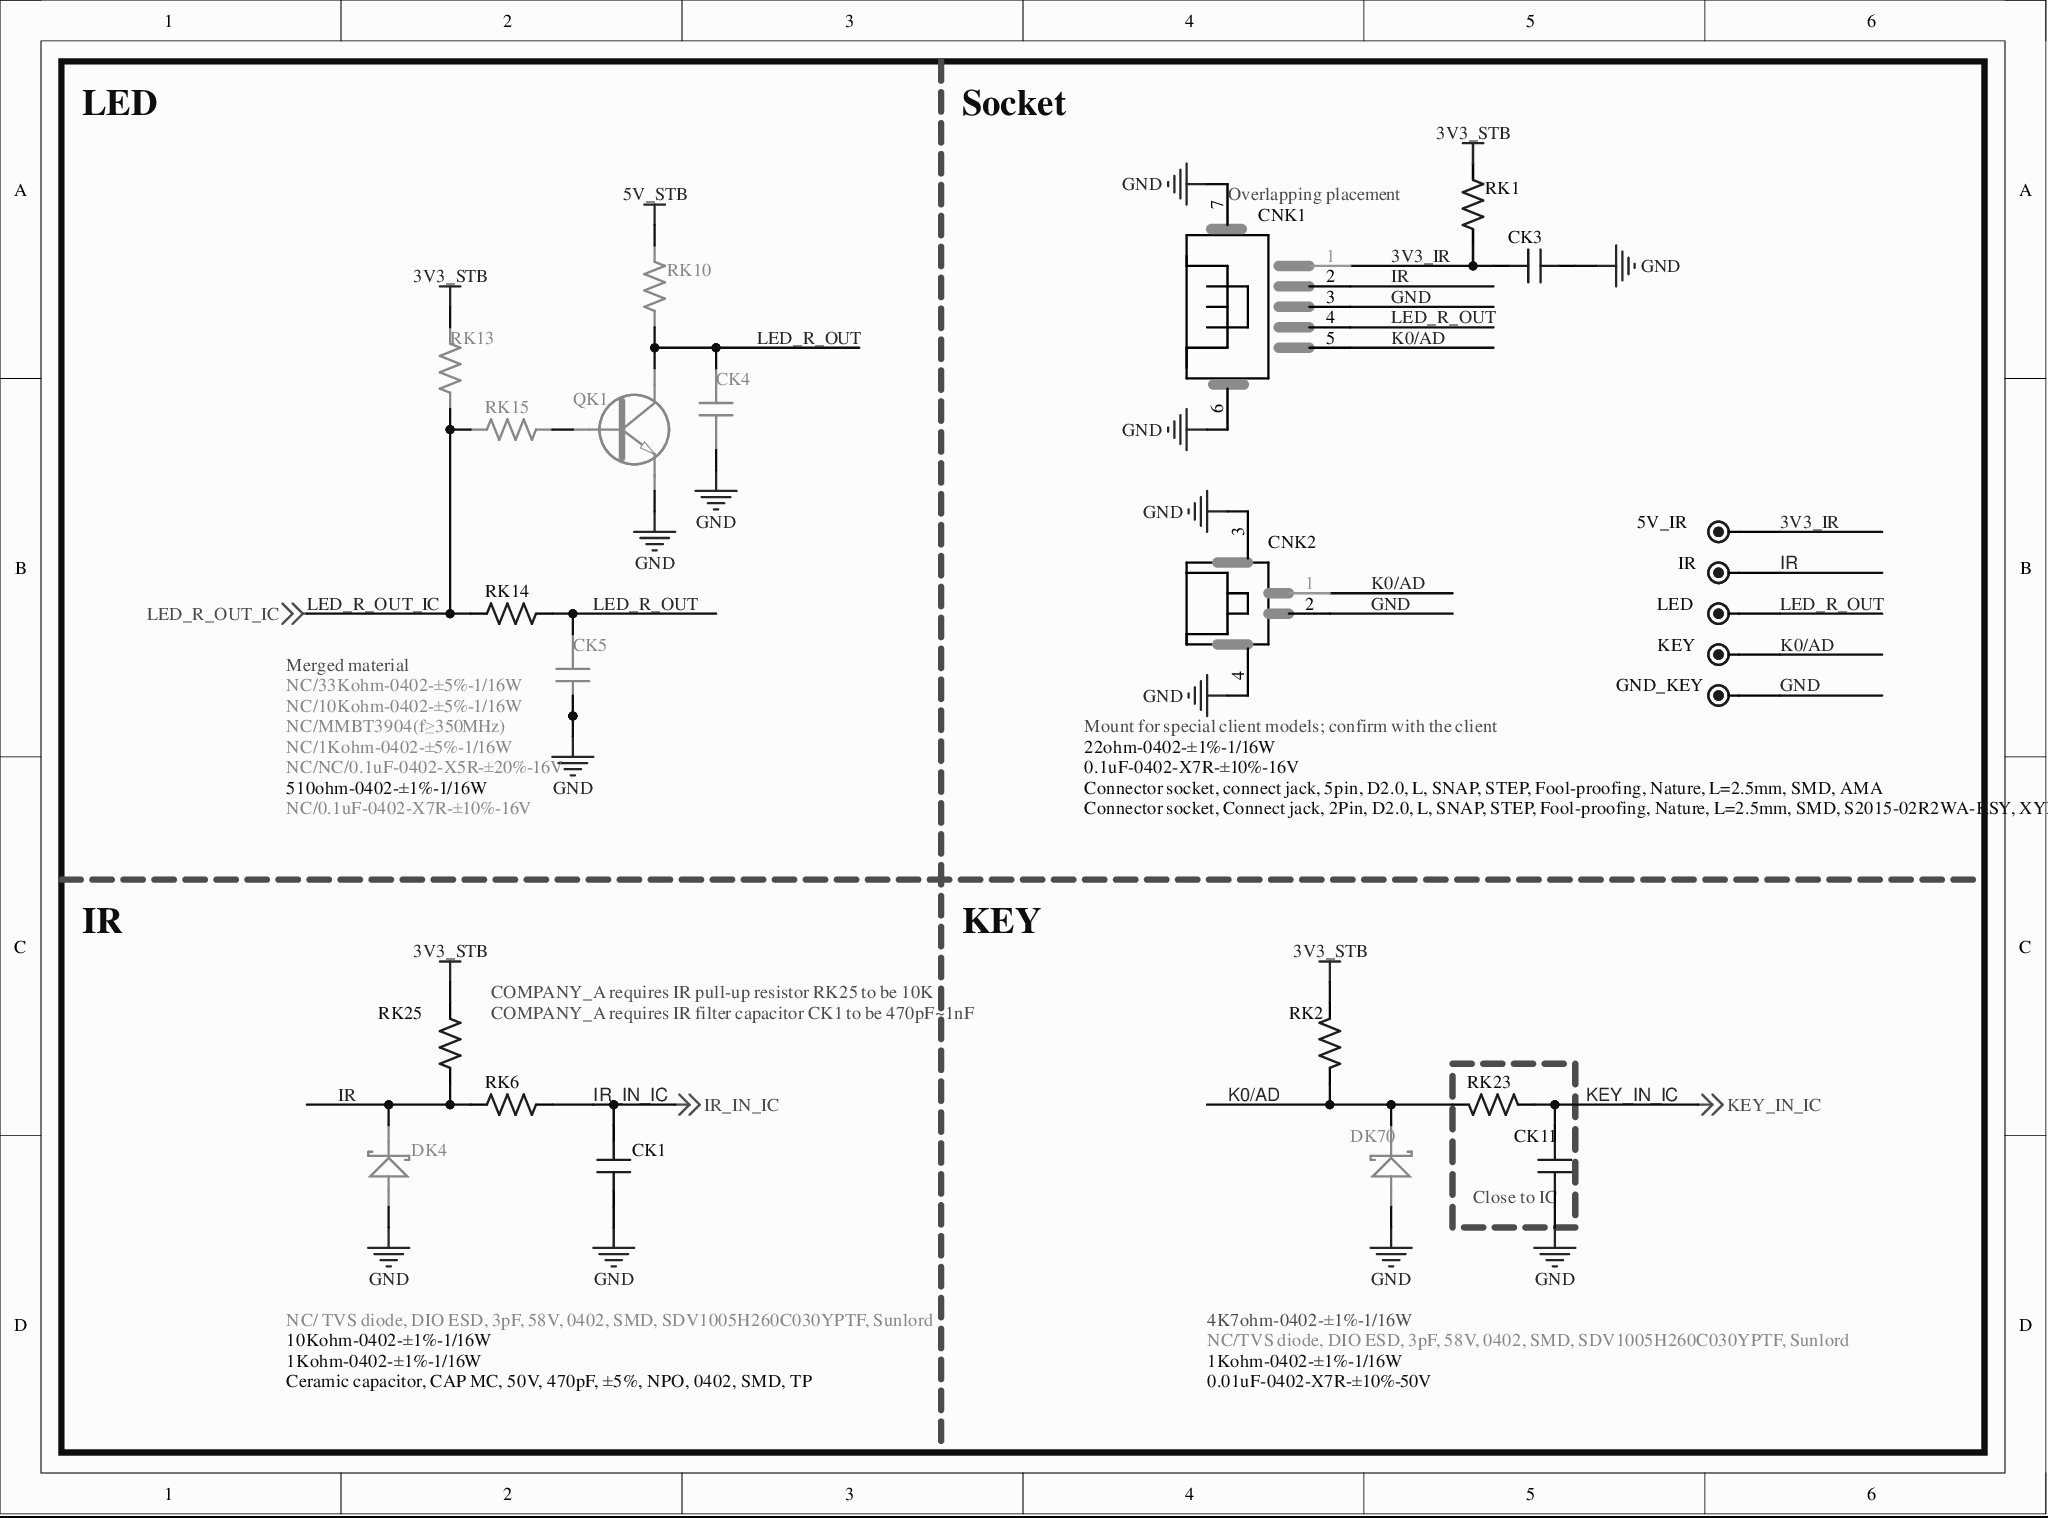
[diagram p0: MISC105950-37.SchDoc]
# Altium project MISC105950-48.PrjPCB (part 5 of 8)

## Sheet MISC105950-37.SchDoc
size 254 x 187 mm

### Parts
5V_IR  DM0  [TP]  (value not drawn)
CK1  Ceramic capacitor, CAP MC, 50V, 470pF, ±5%, NPO, 0402, SMD, TP  [C0402]
CK3  0.1uF-0402-X7R-±10%-16V  [C0402]
CK4  NC/NC/0.1uF-0402-X5R-±20%-16V  [C0402]
CK5  NC/0.1uF-0402-X7R-±10%-16V  [C0402]
CK11  0.01uF-0402-X7R-±10%-50V  [C0402]
CNK1  Connector socket, connect jack, 5pin, D2.0, L, SNAP, STEP, Fool-proofing, Nature, L=2.5mm, SMD, AMA  [SIP5H/2.0S-4]
CNK2  Connector socket, Connect jack, 2Pin, D2.0, L, SNAP, STEP, Fool-proofing, Nature, L=2.5mm, SMD, S2015-02R2WA-KSY, XYDT  [SIP2H/2.0S-3]
DK4  NC/ TVS diode, DIO ESD, 3pF, 58V, 0402, SMD, SDV1005H260C030YPTF, Sunlord  [DIODE-S0402]
DK70  NC/TVS diode, DIO ESD, 3pF, 58V, 0402, SMD, SDV1005H260C030YPTF, Sunlord  [DIODE-S0402]
GND_KEY  DM0  [TP]  (value not drawn)
IR  DM0  [TP]  (value not drawn)
KEY  DM0  [TP]  (value not drawn)
LED  DM0  [TP]  (value not drawn)
QK1  NC/MMBT3904(f≥350MHz)  [SOT-23]
RK1  22ohm-0402-±1%-1/16W  [R0402]
RK2  4K7ohm-0402-±1%-1/16W  [R0402]
RK6  1Kohm-0402-±1%-1/16W  [R0402]
RK10  NC/1Kohm-0402-±5%-1/16W  [R0402]
RK13  NC/33Kohm-0402-±5%-1/16W  [R0402]
RK14  510ohm-0402-±1%-1/16W  [R0402]
RK15  NC/10Kohm-0402-±5%-1/16W  [R0402]
RK23  1Kohm-0402-±1%-1/16W  [R0402]
RK25  10Kohm-0402-±1%-1/16W  [R0402]

### Blocks framed on the sheet
Close to IC: CK11 RK23

### Nets
3V3_STB: RK1.1 RK2.2 RK13.2 RK25.2
5V_STB: RK10.2
GND: CK1.1 CK3.2 CK4.1 CK5.1 CK11.2 CNK1.3 CNK1.6 CNK1.7 CNK2.2 CNK2.3 CNK2.4 DK4.A DK70.A GND_KEY.1 QK1.E
3V3_IR: 5V_IR.1 CK3.1 CNK1.1 RK1.2
IR: CNK1.2 DK4.K IR.1 RK6.1 RK25.1
IR_IN_IC: CK1.2 RK6.2 ; off-sheet IR_IN_IC
K0/AD: CNK1.5 CNK2.1 DK70.K KEY.1 RK2.1 RK23.2
KEY_IN_IC: CK11.1 RK23.1 ; off-sheet KEY_IN_IC
LED_R_OUT: CK4.2 CK5.2 CNK1.4 LED.1 QK1.C RK10.1 RK14.2
LED_R_OUT_IC: RK13.1 RK14.1 RK15.1 ; off-sheet LED_R_OUT_IC
NetQK1_B: QK1.B RK15.2

### Notes on the sheet
- LED
- Socket
- (near CNK1) Overlapping placement
- (near RK14) Merged material
- (near CNK2) Mount for special client models; confirm with the client
- IR
- KEY
- (near RK25) COMPANY_A requires IR filter capacitor CK1 to be 470pF
  nF
- (near RK25) COMPANY_A requires IR pull-up resistor RK25 to be 10K

### Library data of the parts
5V_IR GND_KEY IR KEY LED = TEST
CK1 = 22pF-0402-NPO-±5%-50V-D
CK3 = 0.1uF-0402-Y5V-+80%-20%-16V-D
CK4 CK5 = 004.003.0000403-D: Ceramic capacitor, CAP MC, 16V, 0.1uF, ±20%, X5R, 0402, SMD, TP-D
CK11 = 0.01uF-0402-X7R-±10%-50V-D
CNK1 = XXX.XXX.0001782: Connector socket, connect jack, 5pin, D2.0, L, SNAP, STEP, Fool-proofing, Nature, L=2.5mm, SMD, AMA-D
CNK2 = XXX.XXX.0002231: Connector socket, connect jack, 2Pin, D2.0, L, SNAP, STEP, Fool-proofing, Nature, SMD, 2008-2AW-S, AMA-D
DK4 = AVLC18S02003-D
DK70 = SFI0402-240E-2R5PP-LF-D
QK1 = 004.006.0000007-D: General-purpose transistor, Dynatron, NPN, 0.2A, 40V, 60-300, SOT-23, KMBT3904, KEXIN-D
RK1 = 33ohm-0402-±5%-1/16W-
RK2 = 4K7ohm-0402-±1%-1/16W-D
RK6 RK23 = 1Kohm-0402-±5%-1/16W-D
RK10 = 004.002.0000572-D: Thick-film resistor, RES, 1/16W, 1Kohm, ±5%, 0402, SMD-D
RK13 = 004.002.0000663-D: Thick-film resistor, RES, 1/16W, 33Kohm, ±5%, 0402, SMD-D
RK14 = 004.002.0000699-D: Thick-film resistor, RES, 1/16W, 510ohm, ±1%, 0402, SMD-D
RK15 = 004.002.0000577-D: Thick-film resistor, RES, 1/16W, 10Kohm, ±5%, 0402, SMD-D
RK25 = 4K7ohm-0402-±5%-1/16W-D

## Sheet MISC105950-38.SchDoc
size 368 x 228 mm
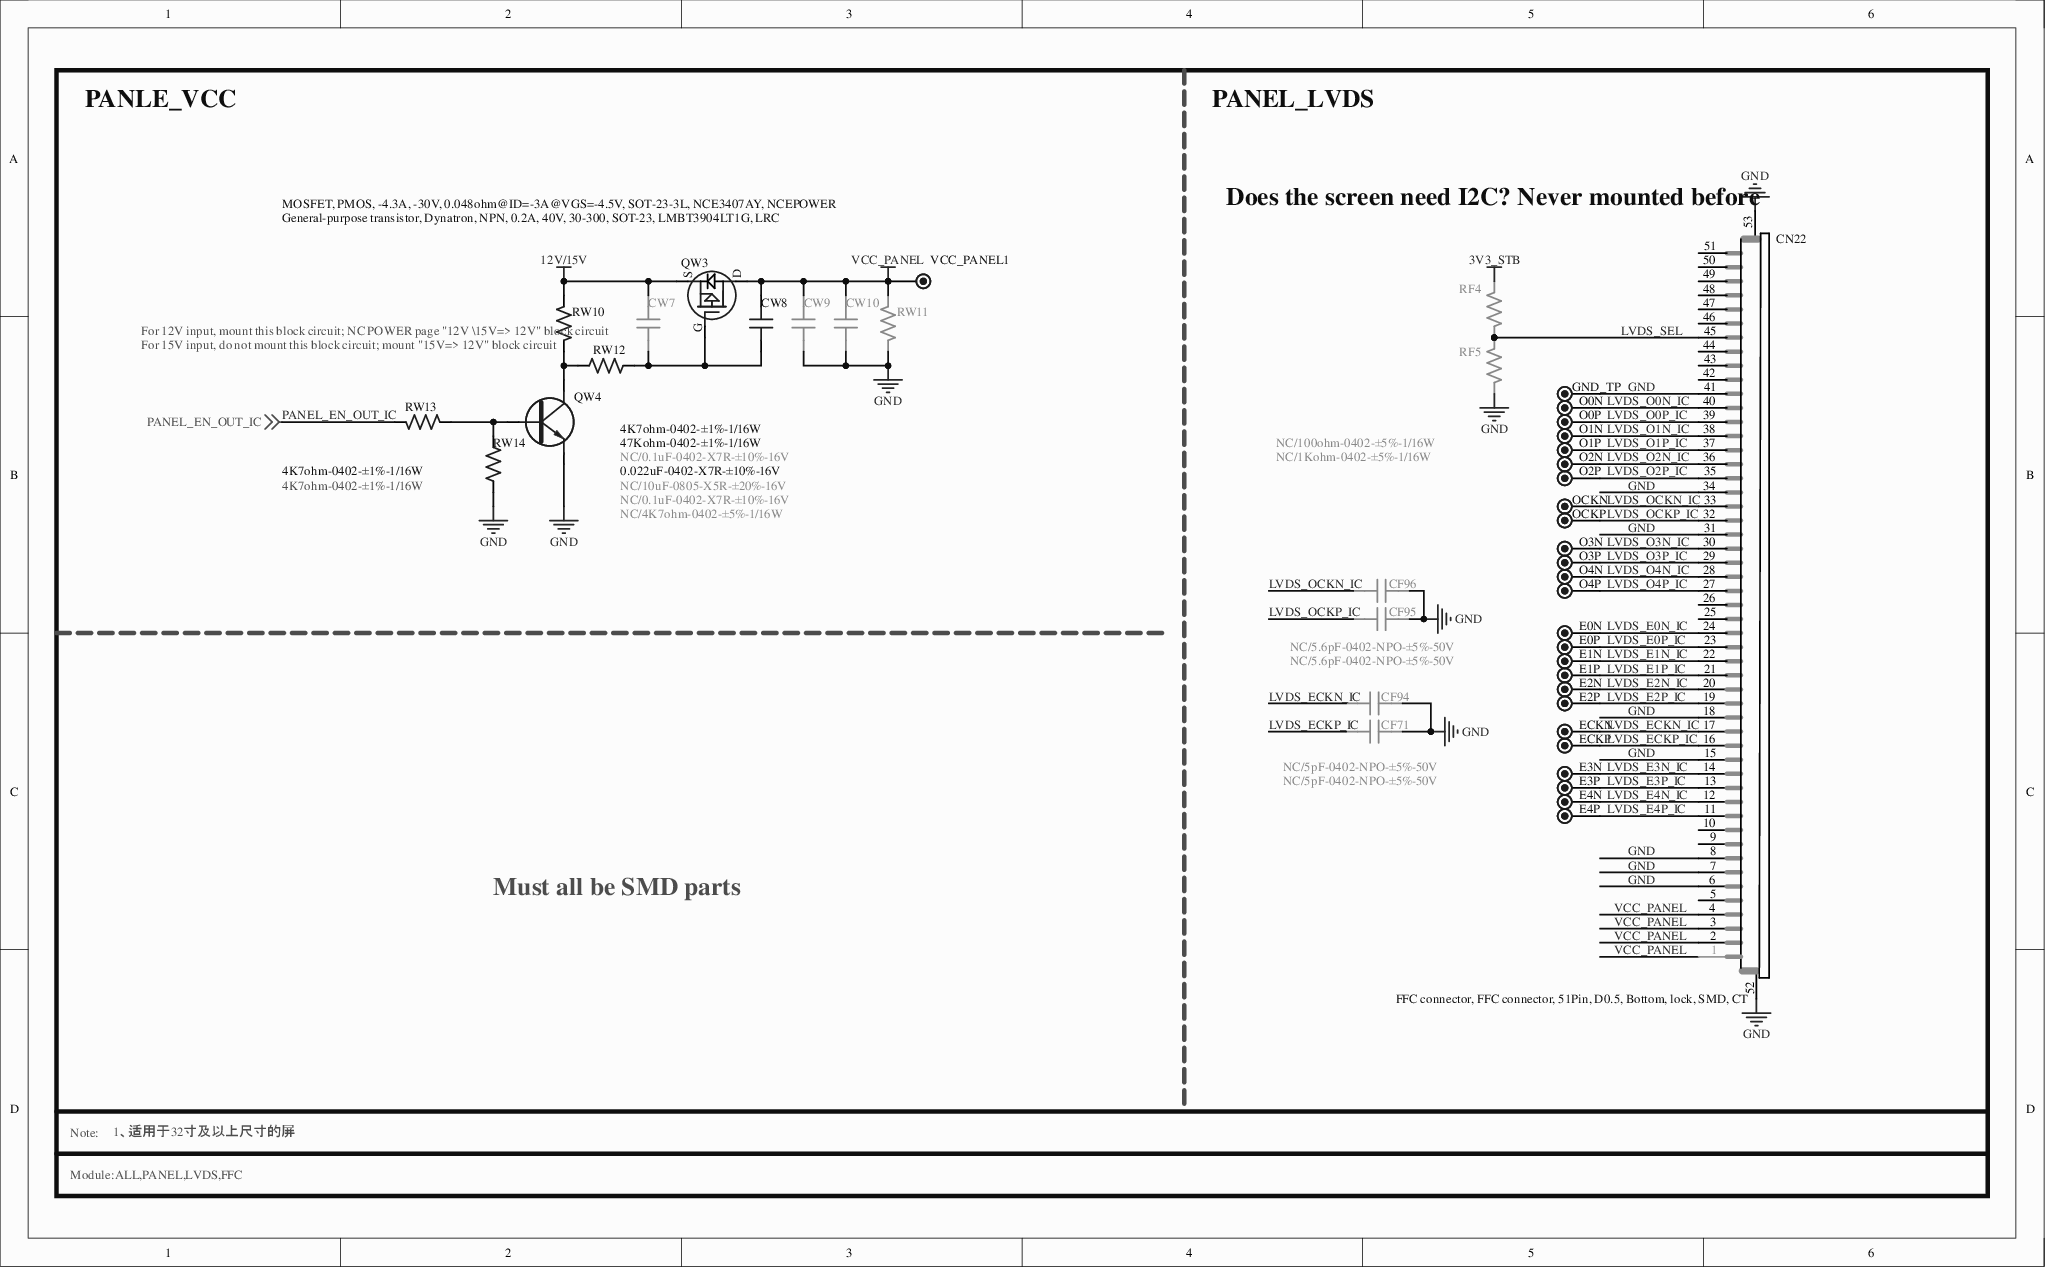
[diagram p1: MISC105950-38.SchDoc]

### Parts
CF71  NC/5pF-0402-NPO-±5%-50V  [C0402]
CF94  NC/5pF-0402-NPO-±5%-50V  [C0402]
CF95  NC/5.6pF-0402-NPO-±5%-50V  [C0402]
CF96  NC/5.6pF-0402-NPO-±5%-50V  [C0402]
CN22  FFC connector, FFC connector, 51Pin, D0.5, Bottom, lock, SMD, CT  [FFC51H/0.5S-8]
CW7  NC/0.1uF-0402-X7R-±10%-16V  [C0402]
CW8  0.022uF-0402-X7R-±10%-16V  [C0402]
CW9  NC/10uF-0805-X5R-±20%-16V  [C0805]
CW10  NC/0.1uF-0402-X7R-±10%-16V  [C0402]
E0N  TEST  [TP]  (value not drawn)
E0P  TEST  [TP]  (value not drawn)
E1N  TEST  [TP]  (value not drawn)
E1P  TEST  [TP]  (value not drawn)
E2N  TEST  [TP]  (value not drawn)
E2P  TEST  [TP]  (value not drawn)
E3N  TEST  [TP]  (value not drawn)
E3P  TEST  [TP]  (value not drawn)
E4N  TEST  [TP]  (value not drawn)
E4P  TEST  [TP]  (value not drawn)
ECKN  TEST  [TP]  (value not drawn)
ECKP  TEST  [TP]  (value not drawn)
GND_TP  TEST  [TP]  (value not drawn)
O0N  TEST  [TP]  (value not drawn)
O0P  TEST  [TP]  (value not drawn)
O1N  TEST  [TP]  (value not drawn)
O1P  TEST  [TP]  (value not drawn)
O2N  TEST  [TP]  (value not drawn)
O2P  TEST  [TP]  (value not drawn)
O3N  TEST  [TP]  (value not drawn)
O3P  TEST  [TP]  (value not drawn)
O4N  TEST  [TP]  (value not drawn)
O4P  TEST  [TP]  (value not drawn)
OCKN  TEST  [TP]  (value not drawn)
OCKP  TEST  [TP]  (value not drawn)
QW3  MOSFET, PMOS, -4.3A, -30V, 0.048ohm@ID=-3A@VGS=-4.5V, SOT-23-3L, NCE3407AY, NCEPOWER  [SOT-23-1]
QW4  General-purpose transistor, Dynatron, NPN, 0.2A, 40V, 30-300, SOT-23, LMBT3904LT1G, LRC  [SOT-23]
RF4  NC/100ohm-0402-±5%-1/16W  [R0402]
RF5  NC/1Kohm-0402-±5%-1/16W  [R0402]
RW10  4K7ohm-0402-±1%-1/16W  [R0402]
RW11  NC/4K7ohm-0402-±5%-1/16W  [R0402]
RW12  47Kohm-0402-±1%-1/16W  [R0402]
RW13  4K7ohm-0402-±1%-1/16W  [R0402]
RW14  4K7ohm-0402-±1%-1/16W  [R0402]
VCC_PANEL1  TEST  [TP]  (value not drawn)

### Nets
3V3_STB: RF4.2
12V/15V: CW7.2 QW3.S RW10.2
GND: CF71.1 CF94.1 CF95.1 CF96.1 CN22.6 CN22.7 CN22.8 CN22.15 CN22.18 CN22.31 CN22.34 CN22.41 CN22.52 CN22.53 CW9.1 CW10.1 GND_TP.1 QW4.E RF5.1 RW11.1 RW14.2
VCC_PANEL: CN22.1 CN22.2 CN22.3 CN22.4 CW8.1 CW9.2 CW10.2 QW3.D RW11.2 VCC_PANEL1.1
LVDS_E0N_IC: CN22.24 E0N.1
LVDS_E0P_IC: CN22.23 E0P.1
LVDS_E1N_IC: CN22.22 E1N.1
LVDS_E1P_IC: CN22.21 E1P.1
LVDS_E2N_IC: CN22.20 E2N.1
LVDS_E2P_IC: CN22.19 E2P.1
LVDS_E3N_IC: CN22.14 E3N.1
LVDS_E3P_IC: CN22.13 E3P.1
LVDS_E4N_IC: CN22.12 E4N.1
LVDS_E4P_IC: CN22.11 E4P.1
LVDS_ECKN_IC: CF94.2 CN22.17 ECKN.1
LVDS_ECKP_IC: CF71.2 CN22.16 ECKP.1
LVDS_O0N_IC: CN22.40 O0N.1
LVDS_O0P_IC: CN22.39 O0P.1
LVDS_O1N_IC: CN22.38 O1N.1
LVDS_O1P_IC: CN22.37 O1P.1
LVDS_O2N_IC: CN22.36 O2N.1
LVDS_O2P_IC: CN22.35 O2P.1
LVDS_O3N_IC: CN22.30 O3N.1
LVDS_O3P_IC: CN22.29 O3P.1
LVDS_O4N_IC: CN22.28 O4N.1
LVDS_O4P_IC: CN22.27 O4P.1
LVDS_OCKN_IC: CF96.2 CN22.33 OCKN.1
LVDS_OCKP_IC: CF95.2 CN22.32 OCKP.1
LVDS_SEL: CN22.45 RF4.1 RF5.2
PANEL_EN_OUT_IC: RW13.1 ; off-sheet PANEL_EN_OUT_IC
NetCW7_1: CW7.1 CW8.2 QW3.G RW12.2
NetQW4_B: QW4.B RW13.2 RW14.1
NetQW4_C: QW4.C RW10.1 RW12.1

Not connected (* = marked no-connect by the designer): CN22 5* 9* 10* 25* 26* 42* 43* 44* 46* 47* 48* 49* 50* 51*

### Notes on the sheet
- PANLE_VCC
- PANEL_LVDS
- (near CN22) Does the screen need I2C? Never mounted before
- For 12V input, mount this block circuit; NC POWER page "12V \15V=> 12V" block circuit
- (near RW10) For 15V input, do not mount this block circuit; mount "15V=> 12V" block circuit
- Must all be SMD parts
- Note:
- 1、适用于32寸及以上尺寸的屏
- Designator range: W1~W50
- Module:ALL,PANEL,LVDS,FFC
- Version:V1.0.0.0

### Library data of the parts
CF71 CF94-CF96 = 5pF-0402-NPO-±5%-50V-D
CN22 = FFC插座,FFC connector,51Pin,D0.5,Bottom,lock,SMD,CT-D: CN-FFC socket, flip-cover
CW7 CW10 = 0.1uF-0402-X5R-±20%-16V-D
CW8 = 0.022uF-0402-X7R-±10%-16V-D
CW9 = 004.003.0000386-D: Ceramic capacitor, CAP MC, 16V, 10uF, ±20%, X5R, 0805, SMD, TP-D
QW3 = 004.007.0000281-D: MOSFET, PMOS, -4.3A, -30V, 0.078ohm@ID=-3A@VGS=-4.5V, SOT-23, AO3487, AOS-D
QW4 = 004.006.0000007-D: as QK1 on sheet MISC105950-37
RF4 = 100ohm-0402-±5%-1/16W-
RF5 = 1Kohm-0402-±5%-1/16W-
RW10 RW11 = 004.002.0000689-D: Thick-film resistor, RES, 1/16W, 4.7Kohm, ±5%, 0402, SMD-D
RW12 = 47Kohm-0402-±5%-1/16W-D
RW13 = 4K7ohm-0402-±5%-1/16W-D
RW14 = 10Kohm-0402-±5%-1/16W-D

## Sheet MISC105950-39.SchDoc
size 441 x 289 mm
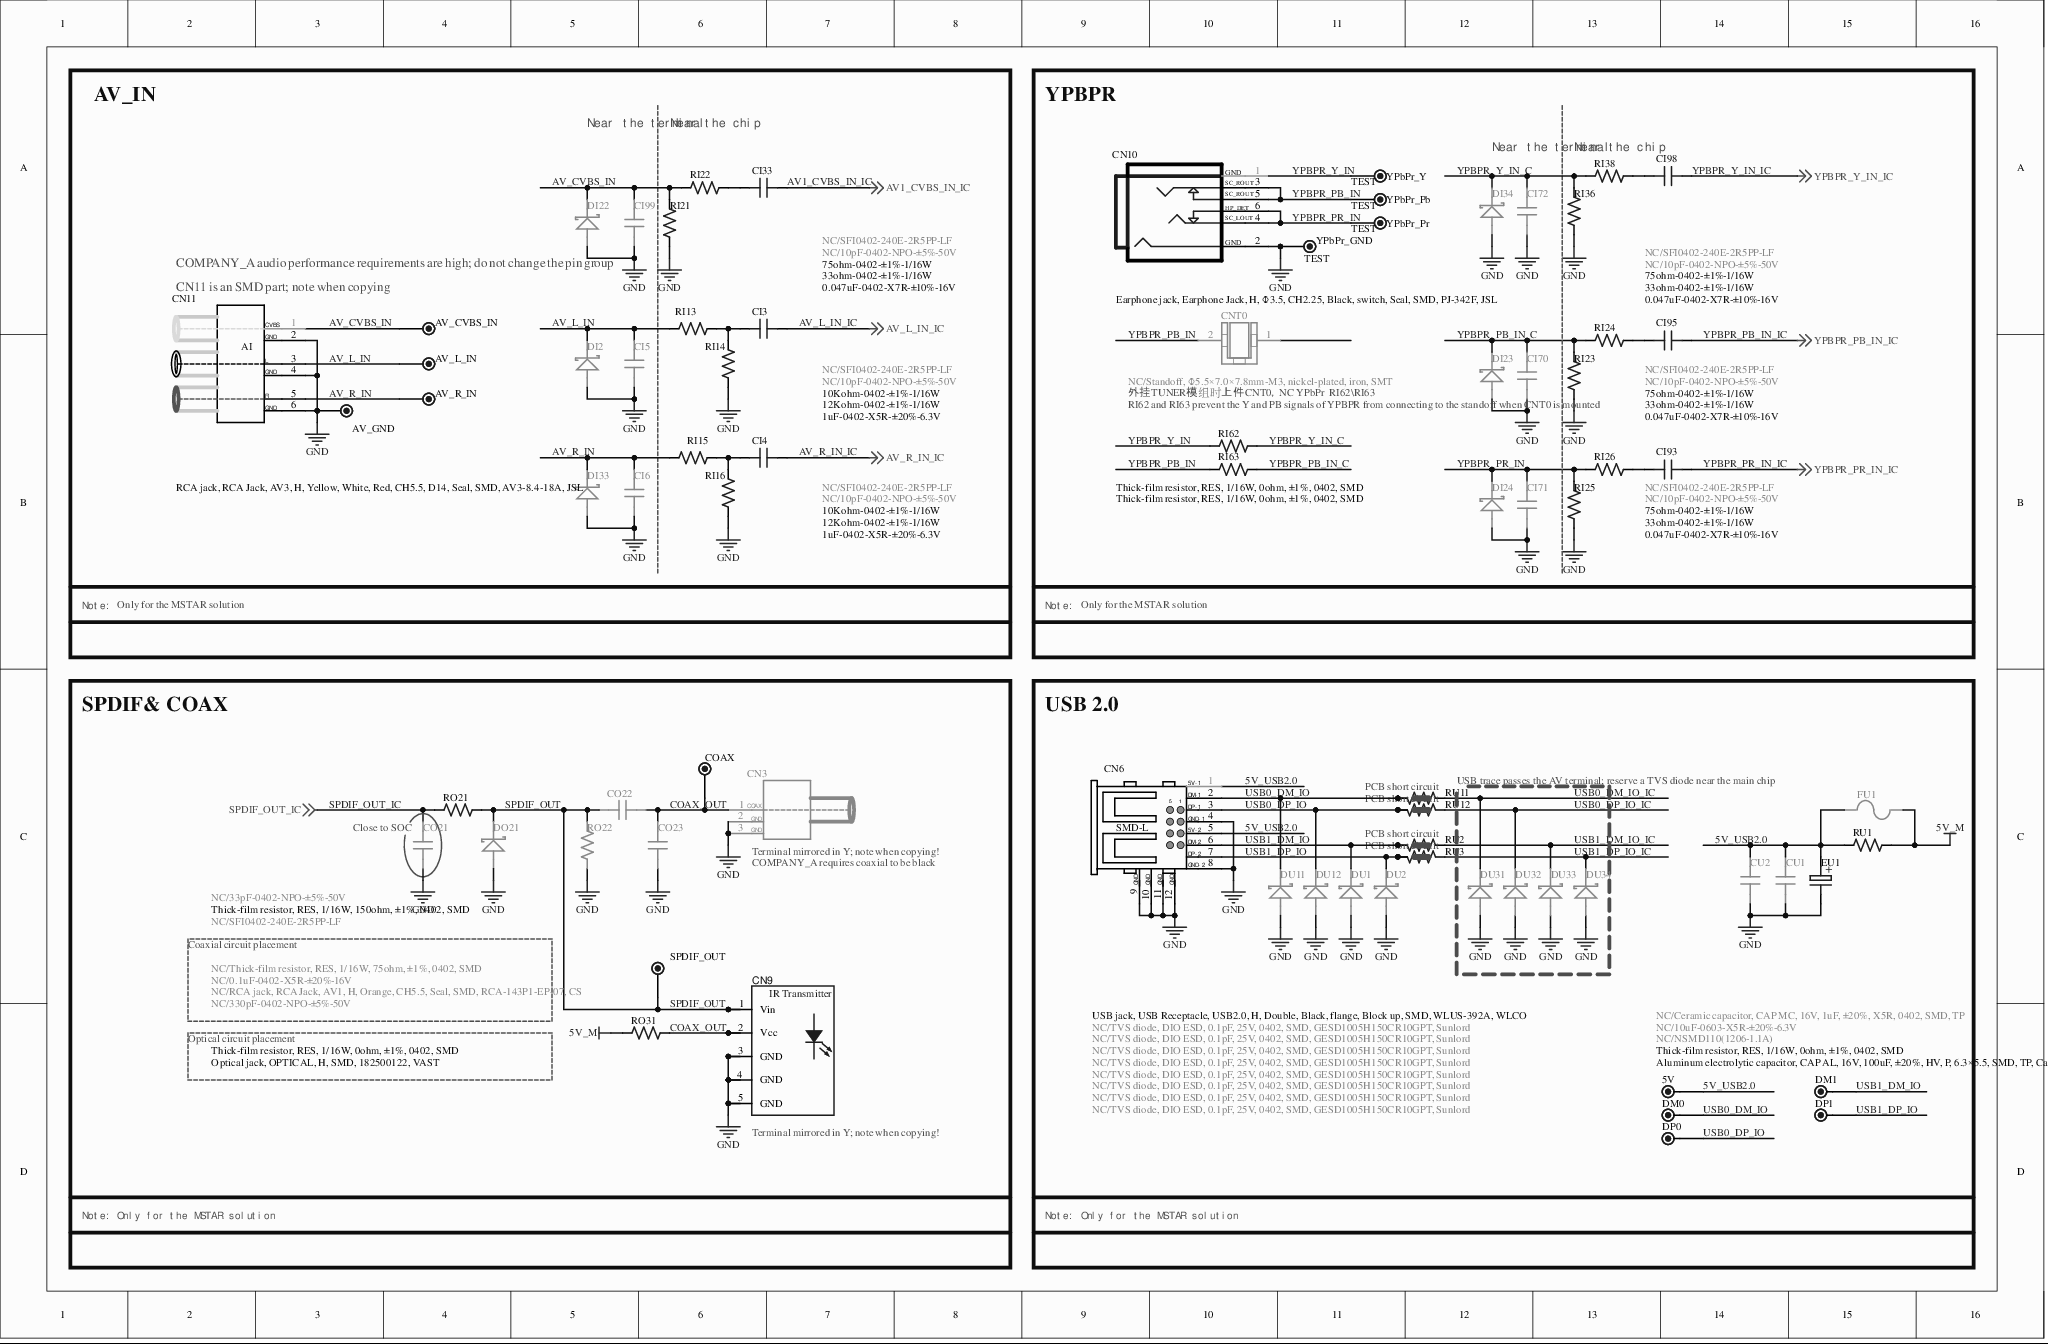
[diagram p2: MISC105950-39.SchDoc]

### Parts
5V  DM0  [TP]  (value not drawn)
AV_CVBS_IN  TEST  [TP]  (value not drawn)
AV_GND  TEST  [TP]  (value not drawn)
AV_L_IN  TEST  [TP]  (value not drawn)
AV_R_IN  TEST  [TP]  (value not drawn)
CI3  1uF-0402-X5R-±20%-6.3V  [C0402]
CI4  1uF-0402-X5R-±20%-6.3V  [C0402]
CI5  NC/10pF-0402-NPO-±5%-50V  [C0402]
CI6  NC/10pF-0402-NPO-±5%-50V  [C0402]
CI33  0.047uF-0402-X7R-±10%-16V  [C0402]
CI70  NC/10pF-0402-NPO-±5%-50V  [C0402]
CI71  NC/10pF-0402-NPO-±5%-50V  [C0402]
CI72  NC/10pF-0402-NPO-±5%-50V  [C0402]
CI93  0.047uF-0402-X7R-±10%-16V  [C0402]
CI95  0.047uF-0402-X7R-±10%-16V  [C0402]
CI98  0.047uF-0402-X7R-±10%-16V  [C0402]
CI99  NC/10pF-0402-NPO-±5%-50V  [C0402]
CN3  NC/RCA jack, RCA Jack, AV1, H, Orange, CH5.5, Seal, SMD, RCA-143P1-EP-07, CS  [AV1-H-4-S]
CN6  USB jack, USB Receptacle, USB2.0, H, Double, Black, flange, Block up, SMD, WLUS-392A, WLCO  [USB2-HS-1]
CN9  Optical jack, OPTICAL, H, SMD, 182500122, VAST  [OPTICAL-HS-1]
CN10  Earphone jack, Earphone Jack, H, Φ3.5, CH2.25, Black, switch, Seal, SMD, PJ-342F, JSL  [PHONE-HS-29]
CN11  RCA jack, RCA Jack, AV3, H, Yellow, White, Red, CH5.5, D14, Seal, SMD, AV3-8.4-18A, JSL  [AV3-H14-15-S]
CNT0  NC/Standoff, Φ5.5×7.0×7.8mm-M3, nickel-plated, iron, SMT  [FIX-5.5*7.0*7.8-S-1]
CO21  NC/33pF-0402-NPO-±5%-50V  [C0402]
CO22  NC/0.1uF-0402-X5R-±20%-16V  [C0402]
CO23  NC/330pF-0402-NPO-±5%-50V  [C0402]
COAX  TEST  [TP]  (value not drawn)
CU1  NC/10uF-0603-X5R-±20%-6.3V  [C0603]
CU2  NC/Ceramic capacitor, CAP MC, 16V, 1uF, ±20%, X5R, 0402, SMD, TP  [C0402]
DI2  NC/SFI0402-240E-2R5PP-LF  [DIODE-S0402]
DI22  NC/SFI0402-240E-2R5PP-LF  [DIODE-S0402]
DI23  NC/SFI0402-240E-2R5PP-LF  [DIODE-S0402]
DI24  NC/SFI0402-240E-2R5PP-LF  [DIODE-S0402]
DI33  NC/SFI0402-240E-2R5PP-LF  [DIODE-S0402]
DI34  NC/SFI0402-240E-2R5PP-LF  [DIODE-S0402]
DM0  DM0  [TP]  (value not drawn)
DM1  DM0  [TP]  (value not drawn)
DO21  NC/SFI0402-240E-2R5PP-LF  [DIODE-S0402]
DP0  DM0  [TP]  (value not drawn)
DP1  DM0  [TP]  (value not drawn)
DU1  NC/TVS diode, DIO ESD, 0.1pF, 25V, 0402, SMD, GESD1005H150CR10GPT, Sunlord  [DIODE-S0402]
DU2  NC/TVS diode, DIO ESD, 0.1pF, 25V, 0402, SMD, GESD1005H150CR10GPT, Sunlord  [DIODE-S0402]
DU11  NC/TVS diode, DIO ESD, 0.1pF, 25V, 0402, SMD, GESD1005H150CR10GPT, Sunlord  [DIODE-S0402]
DU12  NC/TVS diode, DIO ESD, 0.1pF, 25V, 0402, SMD, GESD1005H150CR10GPT, Sunlord  [DIODE-S0402]
DU31  NC/TVS diode, DIO ESD, 0.1pF, 25V, 0402, SMD, GESD1005H150CR10GPT, Sunlord  [DIODE-S0402]
DU32  NC/TVS diode, DIO ESD, 0.1pF, 25V, 0402, SMD, GESD1005H150CR10GPT, Sunlord  [DIODE-S0402]
DU33  NC/TVS diode, DIO ESD, 0.1pF, 25V, 0402, SMD, GESD1005H150CR10GPT, Sunlord  [DIODE-S0402]
DU34  NC/TVS diode, DIO ESD, 0.1pF, 25V, 0402, SMD, GESD1005H150CR10GPT, Sunlord  [DIODE-S0402]
EU1  Aluminum electrolytic capacitor, CAP AL, 16V, 100uF, ±20%, HV, P, 6.3×5.5, SMD, TP, CapXon  [EC(6.5*5.5)-S]
FU1  NC/NSMD110(1206-1.1A)  [FUSE1.1A-S]
RI13  10Kohm-0402-±1%-1/16W  [R0402]
RI14  12Kohm-0402-±1%-1/16W  [R0402]
RI15  10Kohm-0402-±1%-1/16W  [R0402]
RI16  12Kohm-0402-±1%-1/16W  [R0402]
RI21  75ohm-0402-±1%-1/16W  [R0402]
RI22  33ohm-0402-±1%-1/16W  [R0402]
RI23  75ohm-0402-±1%-1/16W  [R0402]
RI24  33ohm-0402-±1%-1/16W  [R0402]
RI25  75ohm-0402-±1%-1/16W  [R0402]
RI26  33ohm-0402-±1%-1/16W  [R0402]
RI36  75ohm-0402-±1%-1/16W  [R0402]
RI38  33ohm-0402-±1%-1/16W  [R0402]
RI62  Thick-film resistor, RES, 1/16W, 0ohm, ±1%, 0402, SMD  [R0402]
RI63  Thick-film resistor, RES, 1/16W, 0ohm, ±1%, 0402, SMD  [R0402]
RO21  Thick-film resistor, RES, 1/16W, 150ohm, ±1%, 0402, SMD  [R0402]
RO22  NC/Thick-film resistor, RES, 1/16W, 75ohm, ±1%, 0402, SMD  [R0402]
RO31  Thick-film resistor, RES, 1/16W, 0ohm, ±1%, 0402, SMD  [R0402]
RU1  Thick-film resistor, RES, 1/16W, 0ohm, ±1%, 0402, SMD  [R0402]
RU2  NC/0ohm-0402-PCB  [R0402SC]  (value not drawn)
RU3  NC/0ohm-0402-PCB  [R0402SC]  (value not drawn)
RU11  NC/0ohm-0402-PCB  [R0402SC]  (value not drawn)
RU12  NC/0ohm-0402-PCB  [R0402SC]  (value not drawn)
SPDIF_OUT  TEST  [TP]  (value not drawn)
YPbPr_GND  TEST  [TP]
YPbPr_Pb  TEST  [TP]
YPbPr_Pr  TEST  [TP]
YPbPr_Y  TEST  [TP]

### Blocks framed on the sheet
AV_IN: AV_CVBS_IN AV_GND AV_L_IN AV_R_IN CI3-CI6 CI33 CI99 CN11 DI2 DI22 DI33 RI13-RI16 RI21 RI22
YPBPR: CI70-CI72 CI93 CI95 CI98 CN10 CNT0 DI23 DI24 DI34 RI23-RI26 RI36 RI38 RI62 RI63 YPbPr_GND YPbPr_Pb YPbPr_Pr YPbPr_Y
SPDIF& COAX: CN3 CN9 CO21-CO23 COAX DO21 RO21 RO22 RO31 SPDIF_OUT
USB 2.0: 5V CN6 CU1 CU2 DM0 DM1 DP0 DP1 DU1 DU2 DU11 DU12 DU31-DU34 EU1 FU1 RU1-RU3 RU11 RU12

### Nets
5V_M: FU1.2 RO31.2 RU1.2
GND: AV_GND.1 CI5.1 CI6.1 CI70.1 CI71.1 CI72.1 CI99.1 CN3.2(GND) CN3.3(GND) CN6.4 CN6.8 CN6.9 CN6.10 CN6.11 CN6.12 CN9.3(GND) CN9.4(GND) CN9.5(GND) CN10.2 CN11.2(GND) CN11.4 CN11.6 CO21.1 CO23.1 CU1.1 CU2.2 DI2.A DI22.A DI23.A DI24.A DI33.A DI34.A DO21.A DU1.A DU2.A DU11.A DU12.A DU31.A DU32.A DU33.A DU34.A EU1.2 RI14.2 RI16.2 RI21.1 RI23.1 RI25.1 RI36.1 RO22.1 YPbPr_GND.1
5V_USB2.0: 5V.1 CN6.1 CN6.5 CU1.2 CU2.1 EU1.1 FU1.1 RU1.1
AV1_CVBS_IN_IC: CI33.2 ; off-sheet AV1_CVBS_IN_IC
AV_CVBS_IN: AV_CVBS_IN.1 CI99.2 CN11.1(R) DI22.K RI21.2 RI22.1
AV_L_IN: AV_L_IN.1 CI5.2 CN11.3 DI2.K RI13.2
AV_L_IN_IC: CI3.1 ; off-sheet AV_L_IN_IC
AV_R_IN: AV_R_IN.1 CI6.2 CN11.5 DI33.K RI15.2
AV_R_IN_IC: CI4.1 ; off-sheet AV_R_IN_IC
COAX_OUT: CN3.1(CVBS) CN9.2(Vcc) CO22.2 CO23.2 COAX.1 RO31.1
SPDIF_OUT: CN9.1(Vin) CO22.1 DO21.K RO21.2 RO22.2 SPDIF_OUT.1
SPDIF_OUT_IC: CO21.2 RO21.1 ; off-sheet SPDIF_OUT_IC
USB0_DM_IO: CN6.2 DM0.1 DU11.K RU11.2 RU11.3
USB0_DM_IO_IC: DU31.K RU11.1
USB0_DP_IO: CN6.3 DP0.1 DU12.K RU12.2 RU12.3
USB0_DP_IO_IC: DU32.K RU12.1
USB1_DM_IO: CN6.6 DM1.1 DU1.K RU2.2 RU2.3
USB1_DM_IO_IC: DU33.K RU2.1
USB1_DP_IO: CN6.7 DP1.1 DU2.K RU3.2 RU3.3
USB1_DP_IO_IC: DU34.K RU3.1
YPBPR_PB_IN: CN10.3 CN10.5 CNT0.2 RI63.2 YPbPr_Pb.1
YPBPR_PB_IN_C: CI70.2 DI23.K RI23.2 RI24.1 RI63.1
YPBPR_PB_IN_IC: CI95.2 ; off-sheet YPBPR_PB_IN_IC
YPBPR_PR_IN: CI71.2 CN10.4 CN10.6 DI24.K RI25.2 RI26.1 YPbPr_Pr.1
YPBPR_PR_IN_IC: CI93.2 ; off-sheet YPBPR_PR_IN_IC
YPBPR_Y_IN: CN10.1 RI62.2 YPbPr_Y.1
YPBPR_Y_IN_C: CI72.2 DI34.K RI36.2 RI38.1 RI62.1
YPBPR_Y_IN_IC: CI98.2 ; off-sheet YPBPR_Y_IN_IC
NetCI3_2: CI3.2 RI13.1 RI14.1
NetCI4_2: CI4.2 RI15.1 RI16.1
NetCI33_1: CI33.1 RI22.2
NetCI93_1: CI93.1 RI26.2
NetCI95_1: CI95.1 RI24.2
NetCI98_1: CI98.1 RI38.2

Not connected (* = marked no-connect by the designer): CNT0 1*

### Notes on the sheet
- Near the terminal
- Near the chip
- (near RI38) Near the terminal
- COMPANY_A audio performance requirements are high; do not change the pin group
- CN11 is an SMD part; note when copying
- 外挂TUNER模组时上件CNT0，NC YPbPr  RI62\RI63
- RI62 and RI63 prevent the Y and PB signals of YPBPR from connecting to the standoff when CNT0 is mounted
- Note:
- Only for the MSTAR solution
- (near CO21) Close to SOC
- USB trace passes the AV terminal; reserve a TVS diode near the main chip
- (near CN3) Terminal mirrored in Y; note when copying!
- (near CN3) COMPANY_A requires coaxial to be black
- Coaxial circuit placement
- Optical circuit placement
- (near CN9) Terminal mirrored in Y; note when copying!

### Library data of the parts
5V DM0 DM1 DP0 DP1 = TEST
CI3 CI4 CO22 = 004.003.0000403-D: as CK4 on sheet MISC105950-37
CI5 CI6 CI70-CI72 CI99 = 004.003.0000500-D: Ceramic capacitor, CAP MC, 50V, 10pF, ±5%, NPO, 0402, SMD, TP-D
CI33 CI93 CI95 CI98 = 004.003.0000562-D: Ceramic capacitor, CAP MC, 16V, 0.047uF, ±10%, X7R, 0402, SMD, TP-D
CN3 = XXX.XXX.0004399-D: RCA jack, RCA Jack, AV1, H, Orange, CH5.5, Seal, SMD, RCA-143P1-EP-07, CS-D
CN6 = PKG-003697/P000082044: USB jack, USB2.0, H, Double, flange, SMD, WLUS-364A, WCLO-D; Revision: *
CN9 = XXX.XXX.0002412: Optical jack, OPTICAL, H, SMD, 182500122, VAST-D
CN10 = XXX.XXX.0004228-D: Earphone jack, Earphone Jack, H, Φ3.5, CH2.25, Black, switch, Seal, SMD, PJ-342F, JSL-D
CN11 = XXX.XXX.0003918-D: RCA jack,RCA Jack,AV3,H,Yellow,White,Red,CH5.5,D14,Seal,SMD-L,AⅤ-8.4-16A yellow/white/red,JSL-D
CNT0 = PKG-004688/P000102833-D: Standoff, Φ5.5×7.0×7.8mm-M3, nickel-plated, iron, SMT-D
CO21 = 004.003.0000546-D: Ceramic capacitor, CAP MC, 50V, 33pF, ±5%, NPO, 0402, SMD, TP-D
CO23 = 004.003.0000045-D: Ceramic capacitor, CAP MC, 50V, 330pF, ±5%, NPO, 0402, SMD, TP-D
CU1 = 004.003.0000383-D: Ceramic capacitor, CAP MC, 6.3V, 10uF, ±20%, X5R, 0603, SMD, TP-D
CU2 = 1uF-0402-X5R-±20%-6.3V-D
DI2 DI22-DI24 DI33 DI34 DO21 = 004.005.0000315-D: TVS diode, DIO ESD, 2.5pF, 200V, 0402, SMD, SFI0402-240E-2R5PP-LF, SFI-D
DU1 DU2 DU11 DU12 DU31-DU34 = 004.005.0000203-D: TVS diode, DIO ESD, 0.2pF, 25V, 0402, SMD, AIES12U020R2, AMOTECH-D
EU1 = 004.003.0000405-D: Aluminum electrolytic capacitor, CAP AL, 16V, 100uF, ±20%, HV, P, 6.3×5.5, SMD, TP, CapXon-D
FU1 = 004.026.0000039-D: Resettable fuse, FUSE PTC, 1.1A, 6V, 1206, SMD, TP, TLC-D
RI13 RI15 = 10Kohm-0402-±5%-1/16W-D
RI14 RI16 = 12Kohm-0402-±5%-1/16W-D
RI21 RI23 RI25 RI36 = 004.002.0000728-D: Thick-film resistor, RES, 1/16W, 75ohm, ±5%, 0402, SMD-D
RI22 RI24 RI26 RI38 = 004.002.0000658-D: Thick-film resistor, RES, 1/16W, 33ohm, ±5%, 0402, SMD-D
RI62 RI63 = 150ohm-0402-±5%-1/16W-D
RO21 = 004.002.0000609-D: Thick-film resistor, RES, 1/16W, 180ohm, ±5%, 0402, SMD-D
RO22 = 004.002.0000568-D: Thick-film resistor, RES, 1/16W, 100ohm, ±5%, 0402, SMD-D
RO31 RU1 = 004.002.0000558-D: Thick-film resistor, RES, 1/16W, 0ohm, ±5%, 0402, SMD-D
RU2 RU3 RU11 RU12 = 0ohm-0402-PCB-D